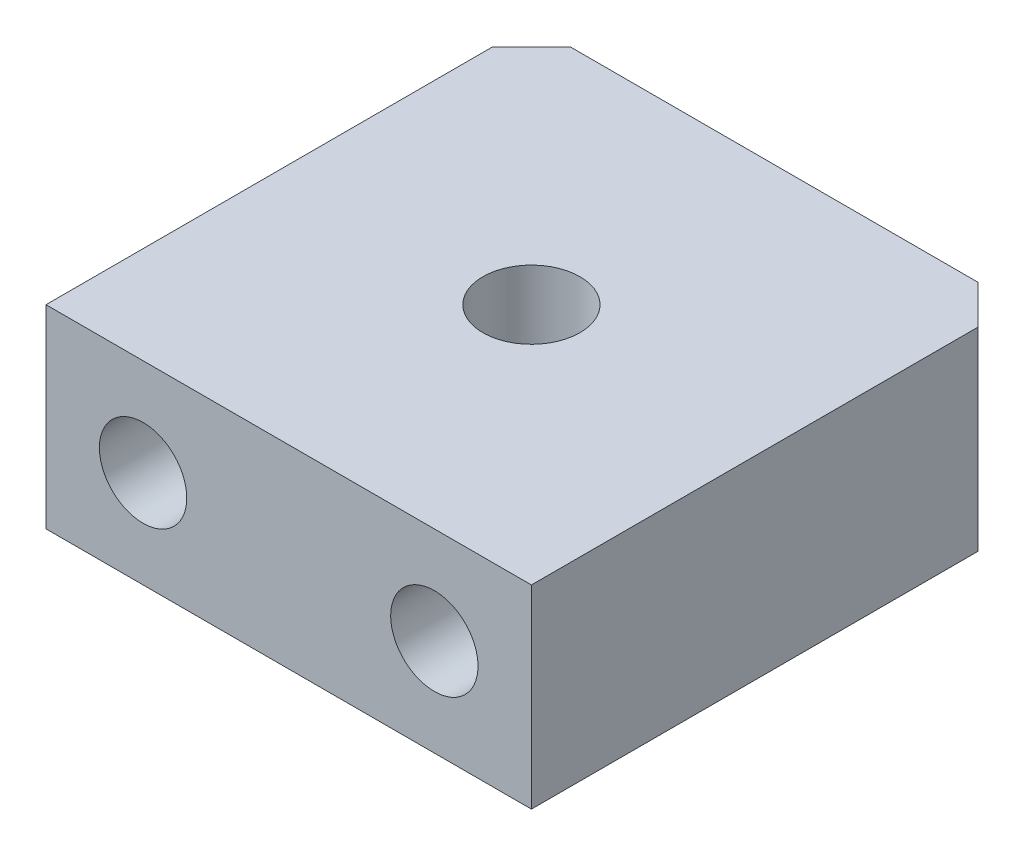
SolidWorks part; units mm, degrees
ref_plane "前视基准面" through (0, 0, 0) normal (0, 0, 1) x (1, 0, 0)
ref_plane "上视基准面" through (0, 0, 0) normal (0, 1, 0) x (1, 0, 0)
ref_plane "右视基准面" through (0, 0, 0) normal (1, 0, 0) x (0, 0, -1)
sketch "草图1" plane through (0, 0, 0) normal (0, 1, 0) x (1, 0, 0)
  line L1 (-12.5, -12.5) -> (12.5, -12.5)
  line L2 (-12.5, -12.5) -> (-12.5, 12.5)
  line L3 (-12.5, 12.5) -> (12.5, 12.5)
  line L4 (12.5, -12.5) -> (12.5, 12.5)
  line L5 (-12.5, -12.5) -> (12.5, 12.5) construction
  line L6 (-12.5, 12.5) -> (12.5, -12.5) construction
  point P0 (0, 0)
  dimension "D1" = 25
  dimension "D2" = 25
extrude "凸台-拉伸1" add sketch "草图1" along normal blind 10
chamfer "倒角1" distance 2 angle 45 2 edges at (-12.5, 5, -12.5) (12.5, 5, -12.5)
sketch "草图4" plane through (0, 0, 0) normal (0, -1, 0) x (-1, 0, 0)
  point P0 (0, 0)
hole_wizard "M6 螺纹孔1" positions "草图4" profile "草图3" tap size "M6" standard "GB" end condition through all
sketch "草图3" plane through (0, 0, 0) normal (1, 0, 0) x (0, 0, -1)
  line L0 (0, 0) -> (0, 10)
  line L1 (0, 10) -> (2.5, 10)
  line L2 (2.5, 10) -> (2.5, 0)
  line L5 (2.5, 0) -> (0, 0)
  line L11 (0, -6.35) -> (0, 107.95) construction
  dimension "通孔螺纹孔钻头直径" = 5
  dimension "通孔螺纹孔钻头深度" = 10
cosmetic thread "孔螺纹线1" parameters "D2"=6
sketch "草图8" plane through (0, 0, -12.5) normal (0, 0, -1) x (-1, 0, 0)
  line L0 (0, 0) -> (0, 17.4246) construction
  line L2 (-12.5, 0) -> (-12.5, 10) construction
  point P0 (-7.5, 5)
  point P8 (7.5, 5)
  point P11 (-12.5, 5)
  dimension "D1" = 15
hole_wizard "M4 六角圆柱头螺钉的柱形沉头孔1" positions "草图8" profile "草图6" counterbore size "M4" standard "GB" end condition through all
sketch "草图6" plane through (7.5, 5, -12.5) normal (1, 0, 0) x (0, 1, 0)
  line L0 (0, 0) -> (0, 25)
  line L1 (0, 25) -> (2.25, 25)
  line L3 (2.25, 25) -> (2.25, 19.6)
  line L4 (2.25, 19.6) -> (4, 19.6)
  line L5 (4, 19.6) -> (4, 0)
  line L7 (4, 0) -> (0, 0)
  line L11 (0, -6.35) -> (0, 107.95) construction
  dimension "通孔孔直径" = 4.5
  dimension "通孔孔深度" = 25
  dimension "柱形沉头孔直径" = 8
  dimension "柱形沉头孔深度" = 19.6
